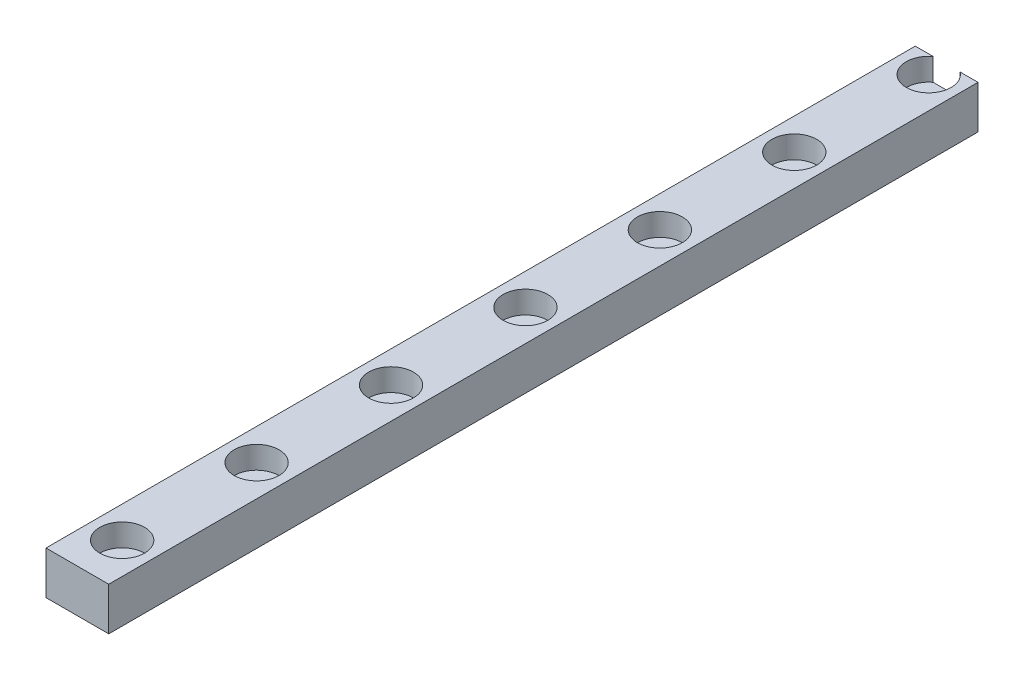
from build123d import *

# Parameters (mm, degrees)
SKETCH1_W           = 7
SKETCH1_H           = 4.8
BOSS_EXTRUDE1_DEPTH = 97
SKETCH2_R           = 1
CUT_EXTRUDE1_DEPTH  = 668
SKETCH3_R           = 2.5
CUT_EXTRUDE2_DEPTH  = 2.5
LPATTERN1_COUNT     = 7
LPATTERN1_PITCH     = 15


with BuildPart() as part:
    # Sketch1 → Boss-Extrude1 (new body)
    with BuildSketch(Plane.XY):
        with Locations((0, 0.250289017)):
            Rectangle(SKETCH1_W, SKETCH1_H)
    extrude(amount=BOSS_EXTRUDE1_DEPTH)

    # Sketch2 → Cut-Extrude1 (cut)
    with BuildSketch(Plane(origin=(0, 2.650289017, 0), x_dir=(1, 0, 0), z_dir=(0, 1, 0))):
        with Locations(Location((0, -92, 0), (0, 0, 270))):
            Circle(SKETCH2_R)
    cut_extrude1 = extrude(amount=-CUT_EXTRUDE1_DEPTH, mode=Mode.SUBTRACT)

    # Sketch3 → Cut-Extrude2 (cut)
    with BuildSketch(Plane(origin=(0, 2.650289017, 0), x_dir=(1, 0, 0), z_dir=(0, 1, 0))):
        with Locations(Location((0, -92, 0), (0, 0, 270))):
            Circle(SKETCH3_R)
    cut_extrude2 = extrude(amount=-CUT_EXTRUDE2_DEPTH, mode=Mode.SUBTRACT)

    # LPattern1: Cut-Extrude1, Cut-Extrude2 ×7
    with Locations(*[(0, 0, -i * LPATTERN1_PITCH) for i in range(1, LPATTERN1_COUNT)]):
        add(cut_extrude1, mode=Mode.SUBTRACT)
        add(cut_extrude2, mode=Mode.SUBTRACT)


solid = part.part
